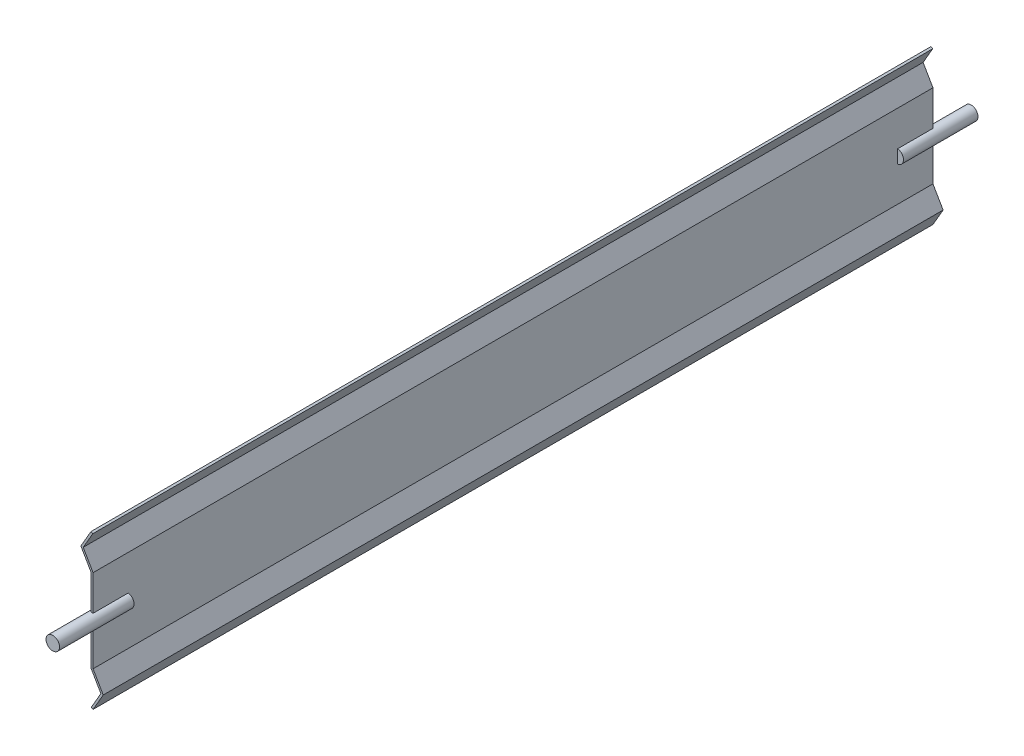
from build123d import *

# Parameters (mm, degrees)
BOSS_EXTRUDE1_DEPTH = 310
BOSS_EXTRUDE2_START = -26
SKETCH2_R           = 5
BOSS_EXTRUDE2_DEPTH = 55


with BuildPart() as part:
    # Sketch1 → Boss-Extrude1 (new, symmetric)
    with BuildSketch(Plane.XY):
        Polygon((0, 0), (7.5, 12.990381057), (0, 25.980762114), (0, 87.421161675), (-7.267949192, 100.009618943), (-0.200961894, 112.25), (-1.5, 113), (-9, 100.009618943), (-1.5, 87.019237886), (-1.5, 25.578838325), (5.767949192, 12.990381057), (-1.299038106, 0.75), align=None)
    extrude(amount=BOSS_EXTRUDE1_DEPTH, both=True)

    # Sketch2 → Boss-Extrude2 (add)
    with BuildSketch(Plane.XY.offset(310).offset(BOSS_EXTRUDE2_START)):
        with Locations((-0.75, 56.5)):
            Circle(SKETCH2_R)
    boss_extrude2 = extrude(amount=BOSS_EXTRUDE2_DEPTH)

    # Mirror1: Boss-Extrude2 across plane
    add(boss_extrude2.mirror(Plane.XY))


solid = part.part
